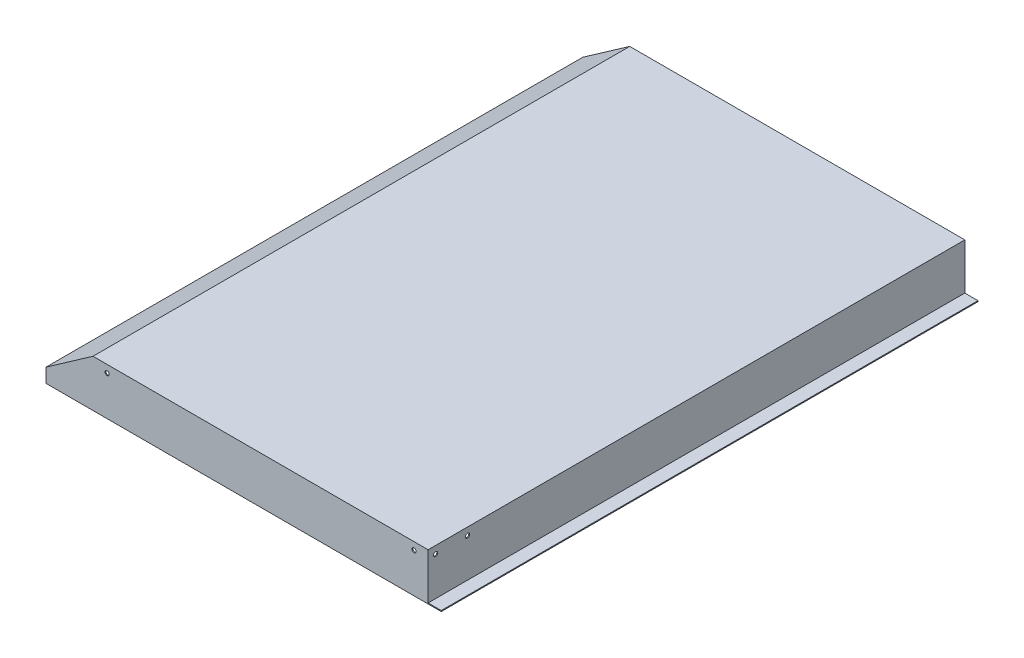
SolidWorks part; units mm, degrees
ref_plane "前视" through (0, 0, 0) normal (0, 0, 1) x (1, 0, 0)
ref_plane "上视" through (0, 0, 0) normal (0, 1, 0) x (1, 0, 0)
ref_plane "右视" through (0, 0, 0) normal (1, 0, 0) x (0, 0, -1)
sketch "草图1" plane through (0, 0, 0) normal (0, 0, 1) x (1, 0, 0)
  line L0 (0, 0) -> (0, 74.115) construction
  line L1 (0, 0) -> (89.4383, 0) construction
  line L2 (0, 0) -> (-813, 0)
  line L3 (-813, 0) -> (-813, 30)
  line L4 (0, 0) -> (0, 100)
  line L5 (0, 100) -> (-713.0296, 100)
  line L6 (-713.0296, 100) -> (-813, 30)
  dimension "D1" = 145
  dimension "D2" = 813
  dimension "D3" = 30
  dimension "D4" = 100
extrude "凸台-拉伸1" add sketch "草图1" along normal mid plane 1142
shell "抽壳1" thickness 2
sketch "草图2" plane through (0, 0, 0) normal (0, -1, 0) x (1, 0, 0)
  line L0 (-813, 571) -> (0, 571) construction
  line L1 (-2, 571) -> (28, 571)
  line L2 (-2, 571) -> (-2, -571)
  line L3 (-2, -571) -> (28, -571)
  line L4 (28, 571) -> (28, -571)
  line L5 (-2, 569) -> (-2, -569) construction
  line L6 (-813, -571) -> (0, -571) construction
extrude "凸台-拉伸2" add sketch "草图2" against normal blind 2
sketch "草图3" plane through (0, 0, 571) normal (0, 0, 1) x (1, 0, 0)
  line L1 (-713.0296, 100) -> (-713.0296, -125.0423) construction
  line L2 (0, 84) -> (-713.0296, 84)
  line L3 (0, 84) -> (-713.0296, 84) construction
  line L4 (-30, 100) -> (-30, -143.1567) construction
  line L5 (0, 100) -> (-713.0296, 100) construction
  line L7 (0, 2) -> (0, 100) construction
  line L8 (-683.0296, 100) -> (-683.0296, -125.0423) construction
  circle A0 centre (-683.0296, 84) radius 4.5
  circle A1 centre (-30, 84) radius 4.5
  dimension "D4" = 9
  dimension "D5" = 9
  dimension "D2" = 30
  dimension "D1" = 16
  dimension "D3" = 30
extrude "切除-拉伸1" cut sketch "草图3" against normal blind 1175
sketch "草图5" plane through (0, 0, 0) normal (0, -1, 0) x (1, 0, 0)
  line L0 (-783, 541) -> (0, 541)
  line L1 (-813, 571) -> (0, 571)
  line L2 (-813, 571) -> (-813, -571)
  line L3 (-813, -571) -> (0, -571)
  line L4 (0, 571) -> (0, 541)
  line L5 (-783, -541) -> (0, -541)
  line L6 (0, -541) -> (0, -571)
  line L7 (-783, 541) -> (-783, -541)
  line L8 (-30, 541) -> (-30, -541) construction
  line L9 (-783, 541) -> (-30, 541) construction
  line L10 (-783, -541) -> (-30, -541) construction
  line L12 (0, 571) -> (0, -571) construction
  dimension "D1" = 30
extrude "凸台-拉伸3" add sketch "草图5" against normal blind 2
sketch "草图6" plane through (0, 0, 0) normal (0, -1, 0) x (1, 0, 0)
  line L1 (28, 0) -> (-1385.4428, 0) construction
  line L2 (-797, -541) -> (-797, 541)
  line L3 (-797, -541) -> (-797, 541) construction
  line L4 (28, -571) -> (28, 571) construction
  line L5 (-813, 571) -> (28, 571) construction
  line L6 (-813, -571) -> (28, -571) construction
  circle A0 centre (-797, 541) radius 4.5
  circle A1 centre (-797, -541) radius 4.5
  circle A2 centre (-797, 0) radius 4.5
  dimension "D2" = 9
  dimension "D3" = 9
  dimension "D4" = 30
  dimension "D5" = 9
  dimension "D6" = 30
  dimension "D1" = 14
extrude "切除-拉伸2" cut sketch "草图6" against normal blind 2
sketch "草图7" plane through (0, 0, 0) normal (1, 0, 0) x (0, 0, -1)
  line L0 (-601.3771, 84) -> (-199.4861, 84) construction
  line L1 (-571, 100) -> (571, 100) construction
  line L2 (-571, 2) -> (-571, 100) construction
  circle A0 centre (-555, 84) radius 4.5
  circle A1 centre (-487, 84) radius 4.5
  dimension "D2" = 9
  dimension "D3" = 9
  dimension "D4" = 16
  dimension "D5" = 68
  dimension "D1" = 16
extrude "切除-拉伸3" cut sketch "草图7" against normal blind 10
